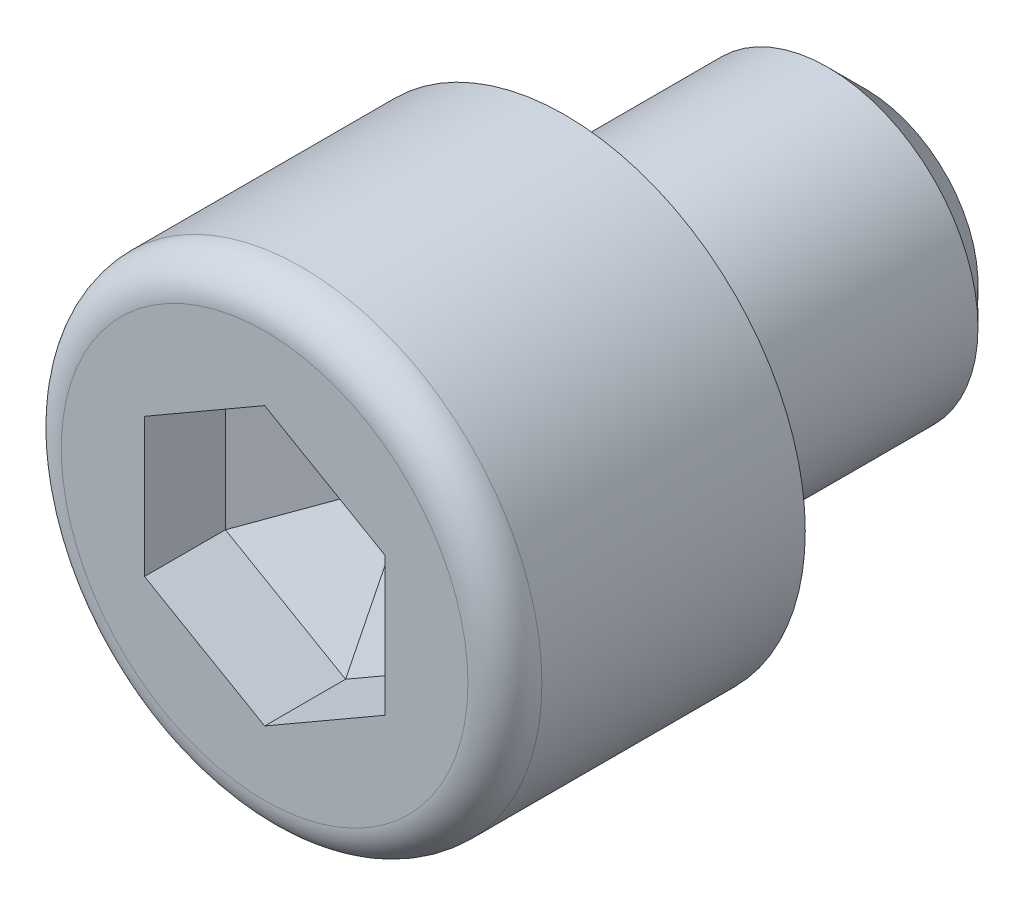
from build123d import *
from OCP.BRepFilletAPI import BRepFilletAPI_MakeChamfer

# Parameters (mm, degrees)
SKETCH_1_R          = 8
EXTRUDE_1_DEPTH     = 10
CUT_EXTRUDE_1_DEPTH = 5
SKETCH_3_R          = 5
EXTRUDE_2_DEPTH     = 10
CHAMFER_1_SIZE      = 1.25
FILLET_1_R          = 1.230769231
CHAMFER_2_SIZE      = 2.305475504
CHAMFER_2_SIZE2     = 3.993200709
FILLET_2_R          = 0.1


with BuildPart() as part:
    # 草图1 → 凸台-拉伸1 (new body)
    with BuildSketch(Plane.XY):
        Circle(SKETCH_1_R)
    extrude(amount=EXTRUDE_1_DEPTH)

    # 草图2 → 切除-拉伸1 (cut)
    with BuildSketch(Plane.XY.offset(10)):
        Polygon((4, 2.309401077), (0, 4.618802154), (-4, 2.309401077), (-4, -2.309401077), (0, -4.618802154), (4, -2.309401077), align=None)
    extrude(amount=-CUT_EXTRUDE_1_DEPTH, mode=Mode.SUBTRACT)

    # 草图3 → 凸台-拉伸2 (add)
    with BuildSketch(Plane(origin=(0, 0, 0), x_dir=(-1, 0, 0), z_dir=(0, 0, -1))):
        with Locations(Location((0, 0, 0), (0, 0, 180))):
            Circle(SKETCH_3_R)
    extrude(amount=EXTRUDE_2_DEPTH)

    # 倒角1
    chamfer_1_edges = [part.edges().sort_by_distance(p)[0] for p in [
        (-5, 0, -10),
    ]]
    chamfer(chamfer_1_edges, length=CHAMFER_1_SIZE)

    # 圆角1
    fillet_1_edges = [part.edges().sort_by_distance(p)[0] for p in [
        (-8, 0, 10),
    ]]
    fillet(fillet_1_edges, radius=FILLET_1_R)

    # 倒角2: one chamfer whose edges measure the first distance from different faces: ONE call of the kernel's chamfer builder (chamfer() names one face for all edges)
    chamfer_2_edges_1 = [part.edges().sort_by_distance(p)[0] for p in [
        (2, 3.464101615, 5),
    ]]
    chamfer_2_side_1 = [part.faces().sort_by_distance(p)[0] for p in [
        (2, 3.464101615, 7.5),
    ]]
    chamfer_2_edges_2 = [part.edges().sort_by_distance(p)[0] for p in [
        (4, 0, 5),
    ]]
    chamfer_2_side_2 = [part.faces().sort_by_distance(p)[0] for p in [
        (4, 0, 7.5),
    ]]
    chamfer_2_edges_3 = [part.edges().sort_by_distance(p)[0] for p in [
        (2, -3.464101615, 5),
    ]]
    chamfer_2_side_3 = [part.faces().sort_by_distance(p)[0] for p in [
        (2, -3.464101615, 7.5),
    ]]
    chamfer_2_edges_4 = [part.edges().sort_by_distance(p)[0] for p in [
        (-2, -3.464101615, 5),
    ]]
    chamfer_2_side_4 = [part.faces().sort_by_distance(p)[0] for p in [
        (-2, -3.464101615, 7.5),
    ]]
    chamfer_2_edges_5 = [part.edges().sort_by_distance(p)[0] for p in [
        (-4, 0, 5),
    ]]
    chamfer_2_side_5 = [part.faces().sort_by_distance(p)[0] for p in [
        (-4, 0, 7.5),
    ]]
    chamfer_2_edges_6 = [part.edges().sort_by_distance(p)[0] for p in [
        (-2, 3.464101615, 5),
    ]]
    chamfer_2_side_6 = [part.faces().sort_by_distance(p)[0] for p in [
        (-2, 3.464101615, 7.5),
    ]]
    chamfer_2 = BRepFilletAPI_MakeChamfer(part.part.solid().wrapped)
    for e in chamfer_2_edges_1:
        chamfer_2.Add(CHAMFER_2_SIZE, CHAMFER_2_SIZE2, e.wrapped, chamfer_2_side_1[0].wrapped)  # the first distance lies on this face
    for e in chamfer_2_edges_2:
        chamfer_2.Add(CHAMFER_2_SIZE, CHAMFER_2_SIZE2, e.wrapped, chamfer_2_side_2[0].wrapped)  # the first distance lies on this face
    for e in chamfer_2_edges_3:
        chamfer_2.Add(CHAMFER_2_SIZE, CHAMFER_2_SIZE2, e.wrapped, chamfer_2_side_3[0].wrapped)  # the first distance lies on this face
    for e in chamfer_2_edges_4:
        chamfer_2.Add(CHAMFER_2_SIZE, CHAMFER_2_SIZE2, e.wrapped, chamfer_2_side_4[0].wrapped)  # the first distance lies on this face
    for e in chamfer_2_edges_5:
        chamfer_2.Add(CHAMFER_2_SIZE, CHAMFER_2_SIZE2, e.wrapped, chamfer_2_side_5[0].wrapped)  # the first distance lies on this face
    for e in chamfer_2_edges_6:
        chamfer_2.Add(CHAMFER_2_SIZE, CHAMFER_2_SIZE2, e.wrapped, chamfer_2_side_6[0].wrapped)  # the first distance lies on this face
    add(Compound.cast(chamfer_2.Shape()), mode=Mode.REPLACE)

    # 圆角2
    fillet_2_edges = [part.edges().sort_by_distance(p)[0] for p in [
        (-5, 0, 0),
    ]]
    fillet(fillet_2_edges, radius=FILLET_2_R)


solid = part.part
